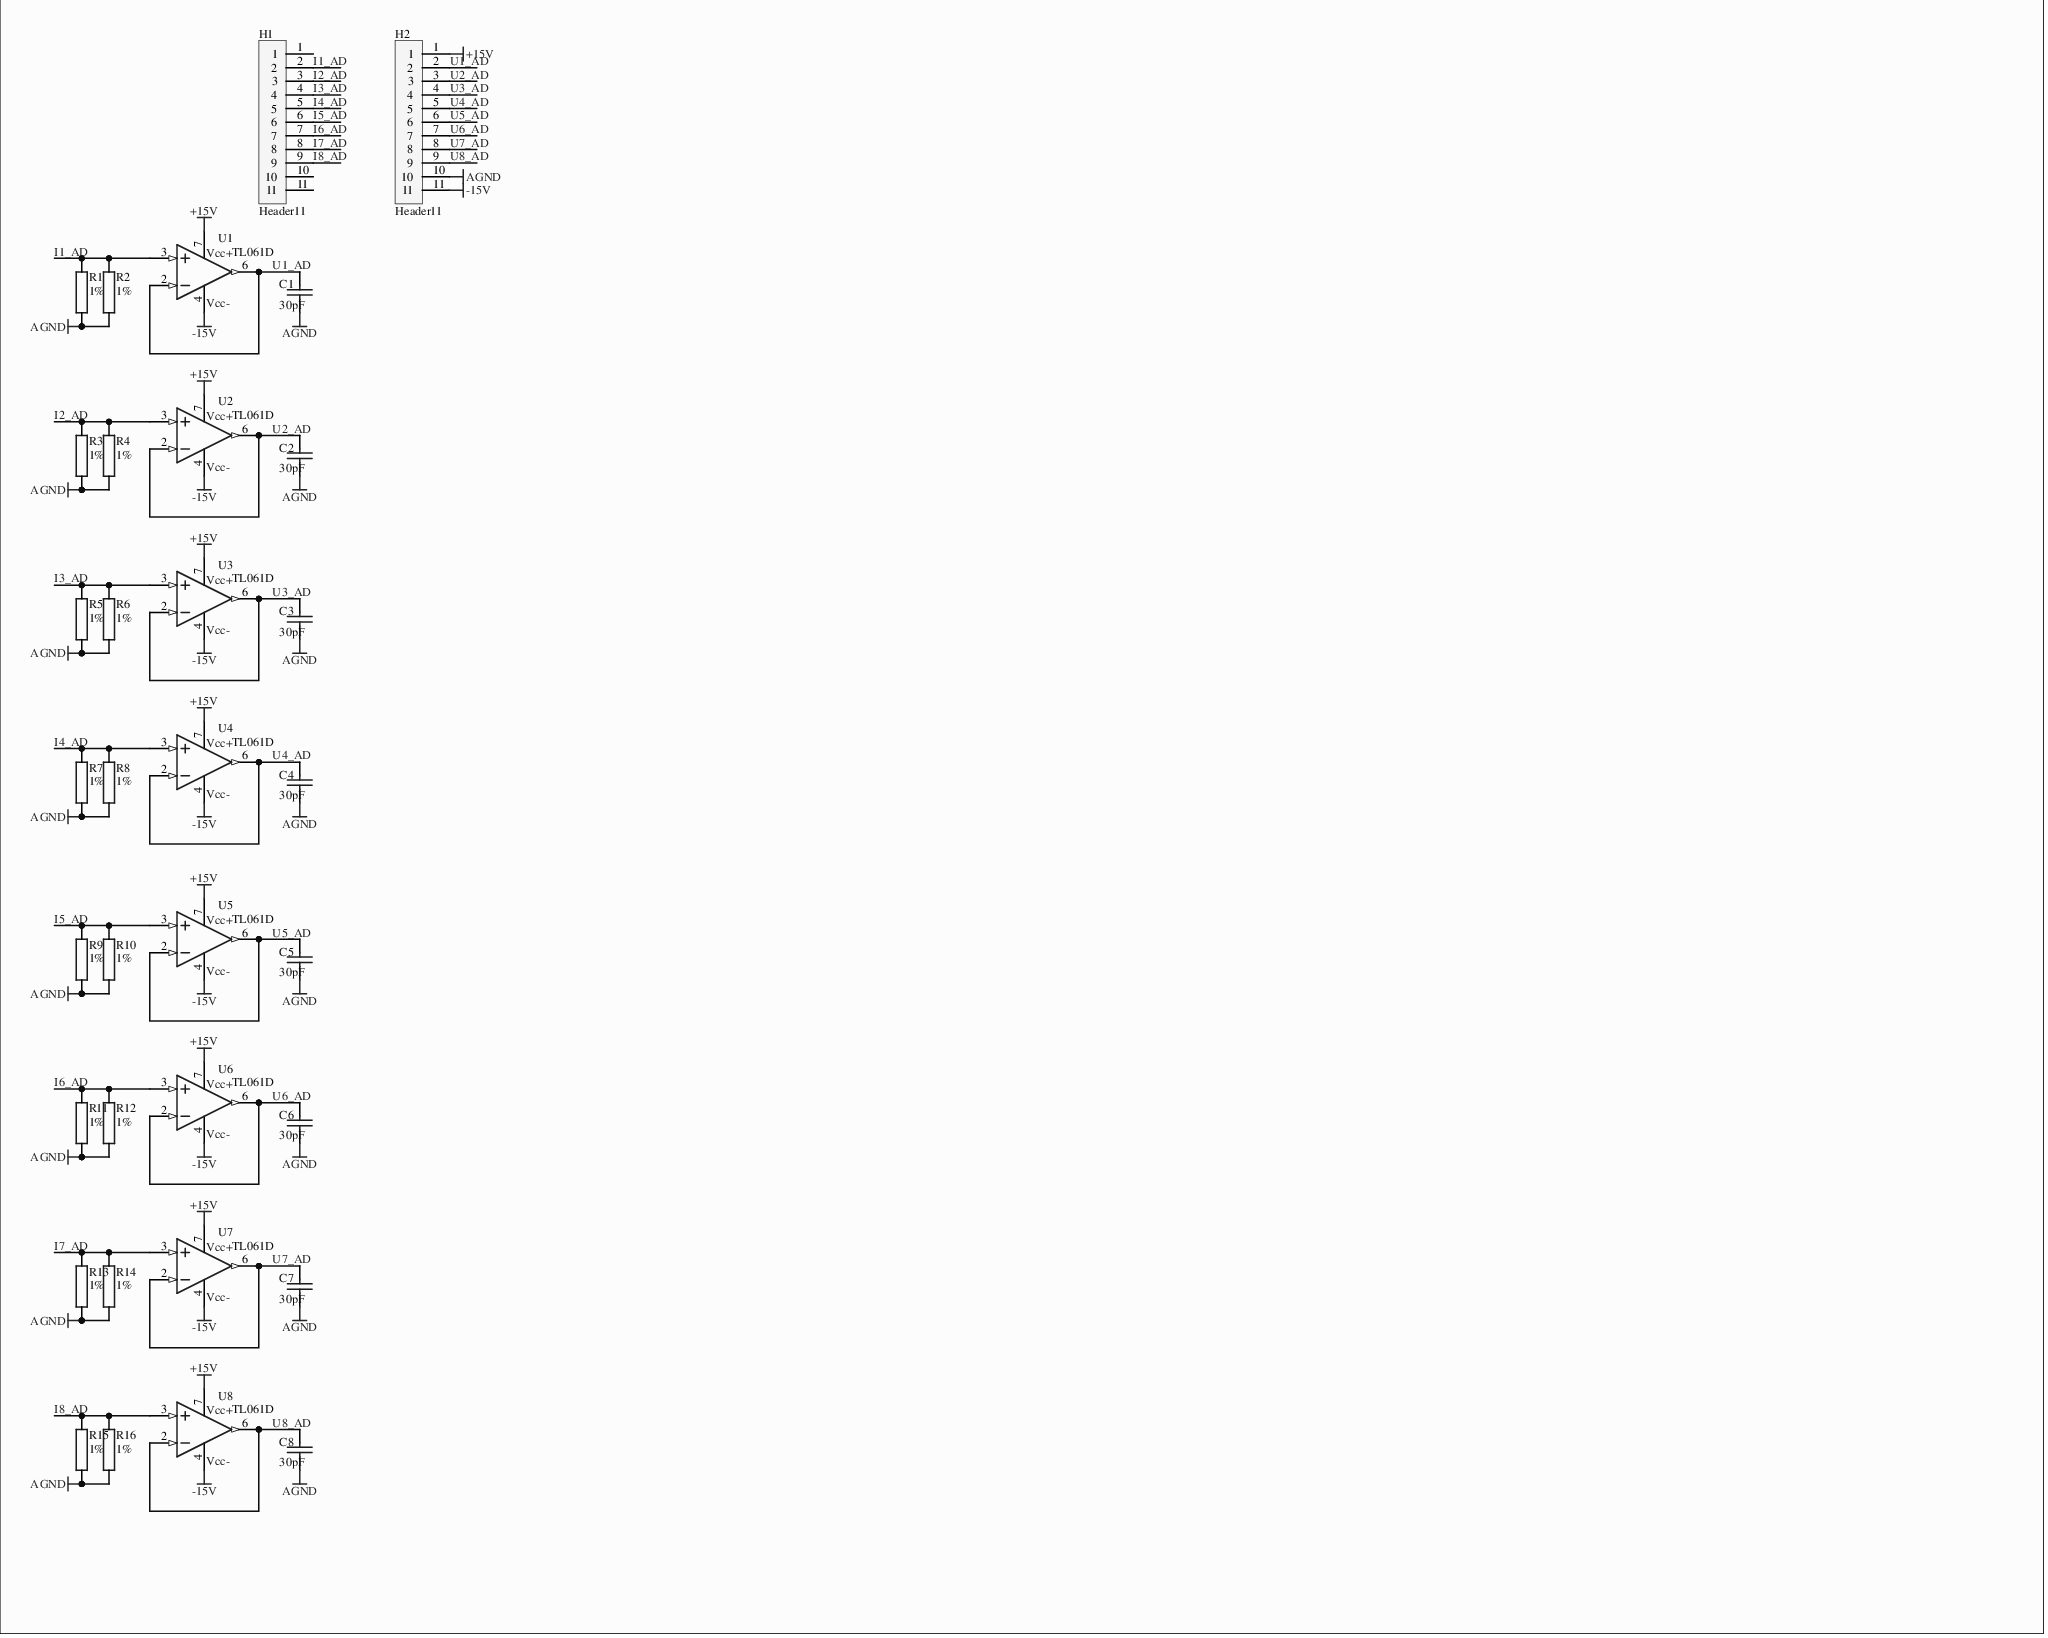
[diagram p0: MISC82250-3.SchDoc]
# Altium project MISC82250-2.PrjPcb
1 sheet, 34 parts. Net scope: global (net labels, ports and power ports of the same name join across sheets).
Board file: MISC82250.PcbDoc

## Sheet MISC82250-3.SchDoc
size 381 x 304 mm

### Parts
C1  30pF  [0603]
C2  30pF  [0603]
C3  30pF  [0603]
C4  30pF  [0603]
C5  30pF  [0603]
C6  30pF  [0603]
C7  30pF  [0603]
C8  30pF  [0603]
H1  Header11  [PinHeader11_1.27mm]
H2  Header11  [PinHeader11_1.27mm]
R1  1%  [1206]
R2  1%  [1206]
R3  1%  [1206]
R4  1%  [1206]
R5  1%  [1206]
R6  1%  [1206]
R7  1%  [1206]
R8  1%  [1206]
R9  1%  [1206]
R10  1%  [1206]
R11  1%  [1206]
R12  1%  [1206]
R13  1%  [1206]
R14  1%  [1206]
R15  1%  [1206]
R16  1%  [1206]
U1  TL061D  [TL061_SOIC8]
U2  TL061D  [TL061_SOIC8]
U3  TL061D  [TL061_SOIC8]
U4  TL061D  [TL061_SOIC8]
U5  TL061D  [TL061_SOIC8]
U6  TL061D  [TL061_SOIC8]
U7  TL061D  [TL061_SOIC8]
U8  TL061D  [TL061_SOIC8]

### Nets
+15V: H2.1 U1.7(V+) U2.7(V+) U3.7(V+) U4.7(V+) U5.7(V+) U6.7(V+) U7.7(V+) U8.7(V+)
-15V: H2.11 U1.4(V-) U2.4(V-) U3.4(V-) U4.4(V-) U5.4(V-) U6.4(V-) U7.4(V-) U8.4(V-)
AGND: C1.1 C2.1 C3.1 C4.1 C5.1 C6.1 C7.1 C8.1 H2.10 R1.2 R2.2 R3.2 R4.2 R5.2 R6.2 R7.2 R8.2 R9.2 R10.2 R11.2 R12.2 R13.2 R14.2 R15.2 R16.2
I1_AD: H1.2 R1.1 R2.1 U1.3(IN+)
I2_AD: H1.3 R3.1 R4.1 U2.3(IN+)
I3_AD: H1.4 R5.1 R6.1 U3.3(IN+)
I4_AD: H1.5 R7.1 R8.1 U4.3(IN+)
I5_AD: H1.6 R9.1 R10.1 U5.3(IN+)
I6_AD: H1.7 R11.1 R12.1 U6.3(IN+)
I7_AD: H1.8 R13.1 R14.1 U7.3(IN+)
I8_AD: H1.9 R15.1 R16.1 U8.3(IN+)
U1_AD: C1.2 H2.2 U1.2(IN-) U1.6(OUT)
U2_AD: C2.2 H2.3 U2.2(IN-) U2.6(OUT)
U3_AD: C3.2 H2.4 U3.2(IN-) U3.6(OUT)
U4_AD: C4.2 H2.5 U4.2(IN-) U4.6(OUT)
U5_AD: C5.2 H2.6 U5.2(IN-) U5.6(OUT)
U6_AD: C6.2 H2.7 U6.2(IN-) U6.6(OUT)
U7_AD: C7.2 H2.8 U7.2(IN-) U7.6(OUT)
U8_AD: C8.2 H2.9 U8.2(IN-) U8.6(OUT)

Not connected (* = marked no-connect by the designer): H1 1* 10* 11*

### Library data of the parts
C1-C8 = CAP: Capacitor
R1-R16 = ProE260.TMP_300K_25